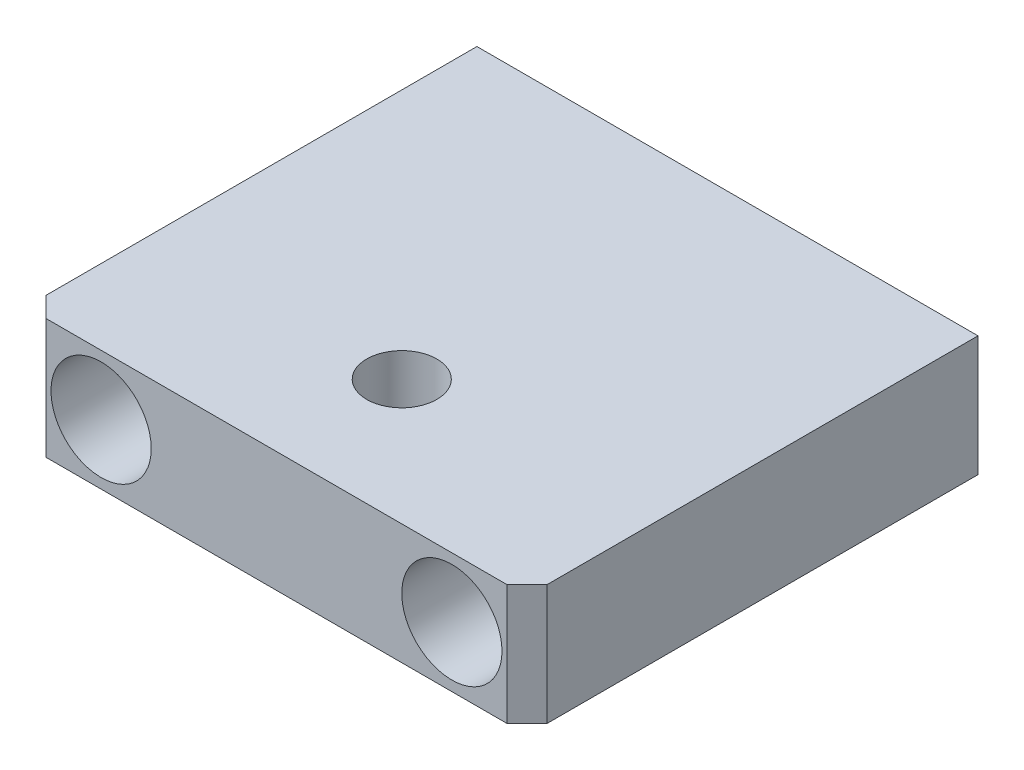
from build123d import *

# Parameters (mm, degrees)
SKETCH1_W                                    = 50
SKETCH1_H                                    = 12
BOSS_EXTRUDE1_DEPTH                          = 22.5
M8X1_0_TAPPED_HOLE1_D                        = 7
HEX_SOCKET_CAP_SCREW_HOLE_TYPE_1_D           = 5.5
HEX_SOCKET_CAP_SCREW_HOLE_TYPE_1_CBORE_D     = 10
HEX_SOCKET_CAP_SCREW_HOLE_TYPE_1_CBORE_DEPTH = 35
CHAMFER1_SIZE                                = 2


with BuildPart() as part:
    # Sketch1 → Boss-Extrude1 (new, symmetric)
    with BuildSketch(Plane.XY):
        Rectangle(SKETCH1_W, SKETCH1_H)
    extrude(amount=BOSS_EXTRUDE1_DEPTH, both=True)

    # M8x1.0 Tapped Hole1 (through all)
    with Locations(Plane(origin=(0, 6, 0), x_dir=(1, 0, 0), z_dir=(0, 1, 0))):
        with Locations((0, -10)):
            Hole(M8X1_0_TAPPED_HOLE1_D / 2)

    # Hex socket cap screw hole type 1 (through all)
    with Locations(Plane.XY.offset(22.5)):
        with Locations((-17.5, 0), (17.5, 0)):
            CounterBoreHole(HEX_SOCKET_CAP_SCREW_HOLE_TYPE_1_D / 2, HEX_SOCKET_CAP_SCREW_HOLE_TYPE_1_CBORE_D / 2, HEX_SOCKET_CAP_SCREW_HOLE_TYPE_1_CBORE_DEPTH)

    # Chamfer1
    chamfer1_edges = [part.edges().sort_by_distance(p)[0] for p in [
        (25, 0, 22.5),
        (-25, 0, 22.5),
    ]]
    chamfer(chamfer1_edges, length=CHAMFER1_SIZE)


solid = part.part
